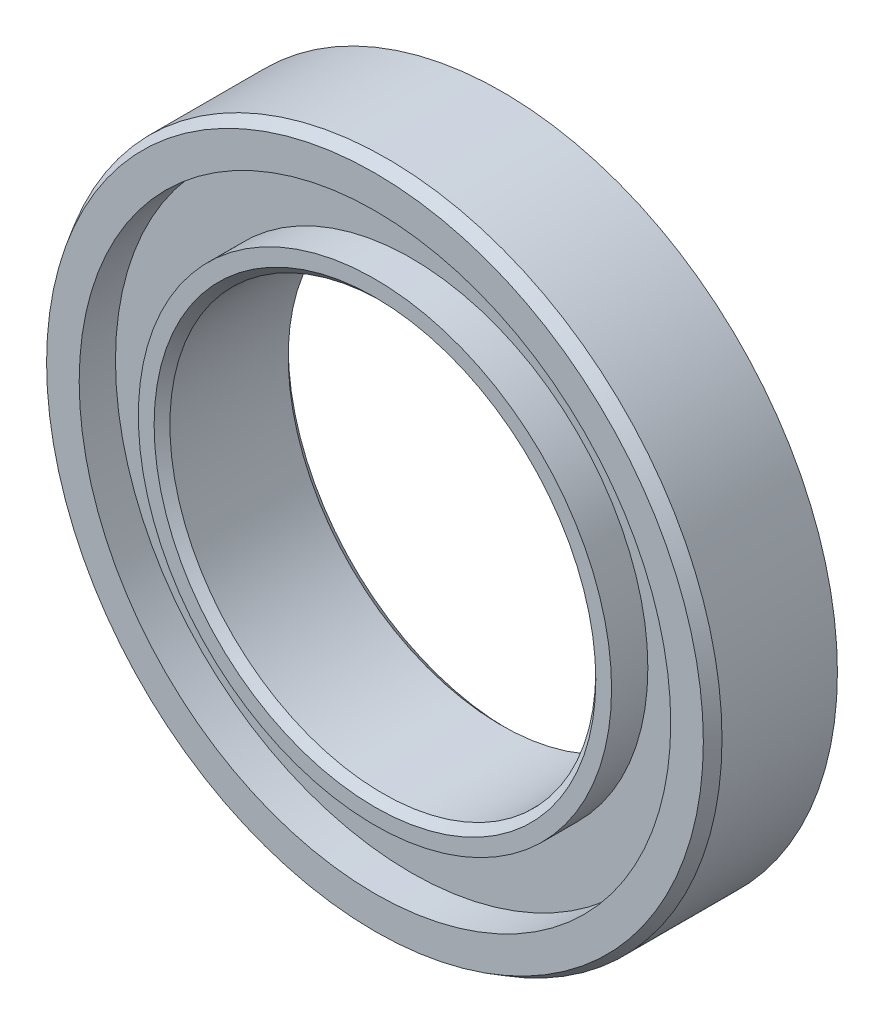
from build123d import *
from OCP.BRepFilletAPI import BRepFilletAPI_MakeChamfer

# Parameters (mm, degrees)
SKETCH1_R           = 42.5
SKETCH1_R_2         = 27
BOSS_EXTRUDE1_DEPTH = 17
SKETCH2_R           = 37.5
SKETCH2_R_2         = 30
CUT_EXTRUDE1_DEPTH  = 4.6
CUT_EXTRUDE2_START  = -4.6
SKETCH3_R           = 37.5
SKETCH3_R_2         = 30
CUT_EXTRUDE2_DEPTH  = 4.6
CHAMFER1_SIZE       = 1.5
CHAMFER1_SIZE2      = 0.866025404
CHAMFER2_SIZE       = 1


with BuildPart() as part:
    # Sketch1 → Boss-Extrude1 (new body)
    with BuildSketch(Plane.XY):
        Circle(SKETCH1_R)
        Circle(SKETCH1_R_2, mode=Mode.SUBTRACT)
    extrude(amount=BOSS_EXTRUDE1_DEPTH)

    # Sketch2 → Cut-Extrude1 (cut)
    with BuildSketch(Plane.XY.offset(17)):
        Circle(SKETCH2_R)
        Circle(SKETCH2_R_2, mode=Mode.SUBTRACT)
    extrude(amount=-CUT_EXTRUDE1_DEPTH, mode=Mode.SUBTRACT)

    # Sketch3 → Cut-Extrude2 (cut)
    with BuildSketch(Plane(origin=(0, 0, 0), x_dir=(-1, 0, 0), z_dir=(0, 0, -1)).offset(CUT_EXTRUDE2_START)):
        with Locations(Location((0, 0, 0), (0, 0, 180))):
            Circle(SKETCH3_R)
        with Locations(Location((0, 0, 0), (0, 0, 180))):
            Circle(SKETCH3_R_2, mode=Mode.SUBTRACT)
    extrude(amount=CUT_EXTRUDE2_DEPTH, mode=Mode.SUBTRACT)

    # Chamfer1: one chamfer whose edges measure the first distance from different faces: ONE call of the kernel's chamfer builder (chamfer() names one face for all edges)
    chamfer1_edges_1 = [part.edges().sort_by_distance(p)[0] for p in [
        (-42.5, 0, 0),
    ]]
    chamfer1_side_1 = [part.faces().sort_by_distance(p)[0] for p in [
        (-41.297918472, 0, 0),
    ]]
    chamfer1_edges_2 = [part.edges().sort_by_distance(p)[0] for p in [
        (-42.5, 0, 17),
    ]]
    chamfer1_side_2 = [part.faces().sort_by_distance(p)[0] for p in [
        (-42.5, 0, 8.5),
    ]]
    chamfer1 = BRepFilletAPI_MakeChamfer(part.part.solid().wrapped)
    for e in chamfer1_edges_1:
        chamfer1.Add(CHAMFER1_SIZE, CHAMFER1_SIZE2, e.wrapped, chamfer1_side_1[0].wrapped)  # the first distance lies on this face
    for e in chamfer1_edges_2:
        chamfer1.Add(CHAMFER1_SIZE, CHAMFER1_SIZE2, e.wrapped, chamfer1_side_2[0].wrapped)  # the first distance lies on this face
    add(Compound.cast(chamfer1.Shape()), mode=Mode.REPLACE)

    # Chamfer2
    chamfer2_edges = [part.edges().sort_by_distance(p)[0] for p in [
        (-27, 0, 0),
        (-27, 0, 17),
    ]]
    chamfer(chamfer2_edges, length=CHAMFER2_SIZE)


solid = part.part
